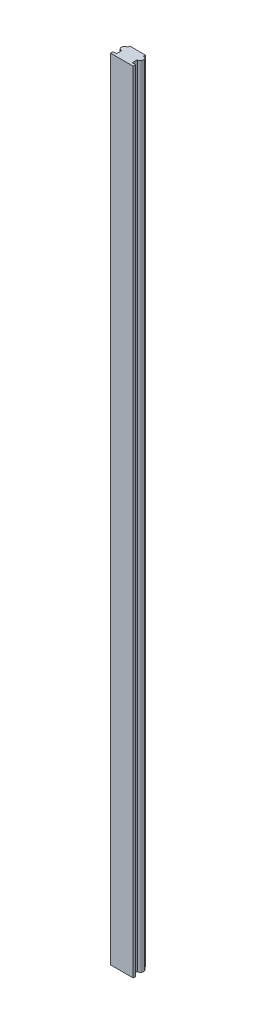
from build123d import *

# Parameters (mm, degrees)
EXTRUDE_1_DEPTH = 1252


with BuildPart() as part:
    # 草图1 → 凸台-拉伸1 (new body)
    with BuildSketch(Plane(origin=(0, 0, 0), x_dir=(1, 0, 0), z_dir=(0, 1, 0))):
        with BuildLine():
            Line((-12.5, 5), (-12.5, 8))
            Line((-12.5, 8), (12.5, 8))
            Line((12.5, 8), (12.5, 5))
            ThreePointArc((12.5, 5), (17.5, 0), (12.5, -5))
            Line((12.5, -5), (12.5, -13))
            Line((12.5, -13), (18, -13))
            Line((18, -13), (18, -17))
            Line((18, -17), (-18, -17))
            Line((-18, -17), (-18, -13))
            Line((-18, -13), (-12.5, -13))
            Line((-12.5, -13), (-12.5, -5))
            ThreePointArc((-12.5, -5), (-17.5, 0), (-12.5, 5))
        make_face()
    extrude(amount=EXTRUDE_1_DEPTH)


solid = part.part
